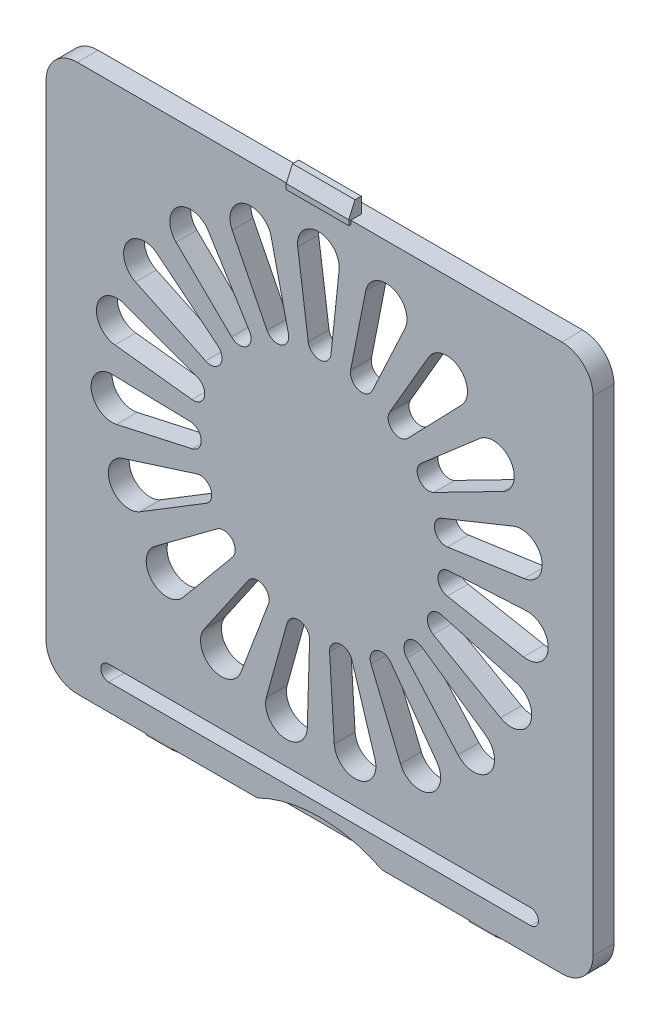
from build123d import *

# Parameters (mm, degrees)
BOSS_EXTRUDE1_DEPTH = 2
CUT_EXTRUDE1_DEPTH  = 12
CUT_EXTRUDE2_START  = -1
SKETCH3_R           = 13.5
CUT_EXTRUDE2_DEPTH  = 1
BOSS_EXTRUDE2_START = 14.25
BOSS_EXTRUDE2_DEPTH = 2.5
BOSS_EXTRUDE3_DEPTH = 3


with BuildPart() as part:
    # Sketch1 → Boss-Extrude1 (new body)
    with BuildSketch(Plane.XY):
        with BuildLine():
            Line((-23.25, 26.25), (23.25, 26.25))
            ThreePointArc((23.25, 26.25), (25.371320344, 25.371320344), (26.25, 23.25))
            Line((26.25, 23.25), (26.25, -23.25))
            ThreePointArc((26.25, -23.25), (25.371320344, -25.371320344), (23.25, -26.25))
            Line((23.25, -26.25), (-23.25, -26.25))
            ThreePointArc((-23.25, -26.25), (-25.371320344, -25.371320344), (-26.25, -23.25))
            Line((-26.25, -23.25), (-26.25, 23.25))
            ThreePointArc((-26.25, 23.25), (-25.371320344, 25.371320344), (-23.25, 26.25))
        make_face()
    extrude(amount=BOSS_EXTRUDE1_DEPTH)

    # Sketch2 → Cut-Extrude1 (cut)
    with BuildSketch(Plane.XY.offset(2)):
        with BuildLine():
            Line((-20.25, -22.25), (20.25, -22.25))
            ThreePointArc((20.25, -22.25), (21, -23), (20.25, -23.75))
            Line((20.25, -23.75), (-20.25, -23.75))
            ThreePointArc((-20.25, -23.75), (-21, -23), (-20.25, -22.25))
        make_face()
        with BuildLine():
            Line((-2.094440492, 21.480216096), (-1.089946345, 14.101618853))
            ThreePointArc((-1.089946345, 14.101618853), (0.01653038, 13.150124213), (1.093913188, 14.134440766))
            Line((1.093913188, 14.134440766), (1.876213205, 21.539892302))
            ThreePointArc((1.876213205, 21.539892302), (-0.1427751, 23.749774158), (-2.094440492, 21.480216096))
        make_face()
        with BuildLine():
            Line((4.425432765, 21.091242282), (2.97967404, 13.786279074))
            ThreePointArc((2.97967404, 13.786279074), (3.717248999, 12.527066633), (5.055863298, 13.108224574))
            Line((5.055863298, 13.108224574), (8.200322325, 19.858415919))
            ThreePointArc((8.200322325, 19.858415919), (7.00827584, 22.604124711), (4.425432765, 21.091242282))
        make_face()
        with BuildLine():
            Line((10.465741714, 18.606344756), (6.726400508, 12.166621695))
            ThreePointArc((6.726400508, 12.166621695), (7.01514601, 10.736146659), (8.469932169, 10.851168508))
            Line((8.469932169, 10.851168508), (13.635799279, 16.21461169))
            ThreePointArc((13.635799279, 16.21461169), (13.399871349, 19.198607267), (10.465741714, 18.606344756))
        make_face()
        with BuildLine():
            Line((15.371925155, 14.294800723), (9.74421711, 9.418161725))
            ThreePointArc((9.74421711, 9.418161725), (9.5528431, 7.971438261), (10.966152465, 7.607859615))
            Line((10.966152465, 7.607859615), (17.593625801, 11.003342342))
            ThreePointArc((17.593625801, 11.003342342), (18.339382876, 13.902262483), (15.371925155, 14.294800723))
        make_face()
        with BuildLine():
            Line((18.612321986, 8.623832879), (11.706096591, 5.838737448))
            ThreePointArc((11.706096591, 5.838737448), (11.055341412, 4.532540491), (12.274019984, 3.729760739))
            Line((12.274019984, 3.729760739), (19.644909973, 4.789329772))
            ThreePointArc((19.644909973, 4.789329772), (21.291537704, 7.289031496), (18.612321986, 8.623832879))
        make_face()
        with BuildLine():
            Line((19.83578493, 2.207978584), (12.399438868, 1.816235025))
            ThreePointArc((12.399438868, 1.816235025), (11.359821941, 0.792111284), (12.251806987, -0.362875933))
            Line((12.251806987, -0.362875933), (19.567363328, -1.754041339))
            ThreePointArc((19.567363328, -1.754041339), (21.93642405, 0.0755605), (19.83578493, 2.207978584))
        make_face()
        with BuildLine():
            Line((18.909732793, -4.257504797), (11.749109546, -2.21344499))
            ThreePointArc((11.749109546, -2.21344499), (10.433289497, -2.844515818), (10.901920596, -4.226549712))
            Line((10.901920596, -4.226549712), (17.369389247, -7.917695201))
            ThreePointArc((17.369389247, -7.917695201), (20.204158471, -6.956458994), (18.909732793, -4.257504797))
        make_face()
        with BuildLine():
            Line((15.934517692, -10.071981817), (9.825581899, -5.813624241))
            ThreePointArc((9.825581899, -5.813624241), (8.376148247, -5.98325584), (8.370641949, -7.442571595))
            Line((8.370641949, -7.442571595), (13.289172328, -13.033704277))
            ThreePointArc((13.289172328, -13.033704277), (16.282458822, -13.044998562), (15.934517692, -10.071981817))
        make_face()
        with BuildLine():
            Line((11.232550351, -14.60536367), (6.837299994, -8.594167444))
            ThreePointArc((6.837299994, -8.594167444), (5.411321364, -8.283977597), (4.932274362, -9.662435707))
            Line((4.932274362, -9.662435707), (7.768867384, -16.547669603))
            ThreePointArc((7.768867384, -16.547669603), (10.596302111, -17.530270468), (11.232550351, -14.60536367))
        make_face()
        with BuildLine():
            Line((5.313361888, -17.36638809), (3.108090542, -10.253759599))
            ThreePointArc((3.108090542, -10.253759599), (1.860093847, -9.497362189), (0.959418316, -10.645585329))
            Line((0.959418316, -10.645585329), (1.406685112, -18.078798509))
            ThreePointArc((1.406685112, -18.078798509), (3.761871648, -19.926225904), (5.313361888, -17.36638809))
        make_face()
        with BuildLine():
            Line((-1.181611781, -18.055855239), (-0.957928747, -10.612558143))
            ThreePointArc((-0.957928747, -10.612558143), (-1.892703701, -9.491920567), (-3.117405592, -10.285480943))
            Line((-3.117405592, -10.285480943), (-5.107933318, -17.461169421))
            ThreePointArc((-5.107933318, -17.461169421), (-3.48021598, -19.973225922), (-1.181611781, -18.055855239))
        make_face()
        with BuildLine():
            Line((-7.548539479, -16.599050654), (-4.920141592, -9.631681687))
            ThreePointArc((-4.920141592, -9.631681687), (-5.440397435, -8.268242415), (-6.856410232, -8.621145447))
            Line((-6.856410232, -8.621145447), (-11.069027916, -14.761712035))
            ThreePointArc((-11.069027916, -14.761712035), (-10.345168205, -17.666177341), (-7.548539479, -16.599050654))
        make_face()
        with BuildLine():
            Line((-13.097465797, -13.153841715), (-8.349180752, -7.417423416))
            ThreePointArc((-8.349180752, -7.417423416), (-8.39853969, -5.958932248), (-9.852416435, -5.832935417))
            Line((-9.852416435, -5.832935417), (-15.830621585, -10.272954444))
            ThreePointArc((-15.830621585, -10.272954444), (-16.089060933, -13.255084672), (-13.097465797, -13.153841715))
        make_face()
        with BuildLine():
            Line((-17.227078467, -8.09357027), (-10.873456626, -4.209732571))
            ThreePointArc((-10.873456626, -4.209732571), (-10.446569853, -2.814239656), (-11.780760442, -2.222996673))
            Line((-11.780760442, -2.222996673), (-18.876721768, -4.481323183))
            ThreePointArc((-18.876721768, -4.481323183), (-20.089454262, -7.217958251), (-17.227078467, -8.09357027))
        make_face()
        with BuildLine():
            Line((-19.48986988, -1.966595247), (-12.219424756, -0.356212226))
            ThreePointArc((-12.219424756, -0.356212226), (-11.362552077, 0.825059124), (-12.432476257, 1.817477908))
            Line((-12.432476257, 1.817477908), (-19.877236245, 1.985568633))
            ThreePointArc((-19.877236245, 1.985568633), (-21.912843501, -0.209014401), (-19.48986988, -1.966595247))
        make_face()
        with BuildLine():
            Line((-19.640631475, 4.56313054), (-12.24122861, 3.725548894))
            ThreePointArc((-12.24122861, 3.725548894), (-11.047225476, 4.564589601), (-11.73694036, 5.85064021))
            Line((-11.73694036, 5.85064021), (-18.723743748, 8.426932933))
            ThreePointArc((-18.723743748, 8.426932933), (-21.361636134, 7.012219056), (-19.640631475, 4.56313054))
        make_face()
        with BuildLine():
            Line((-17.663025894, 10.788009983), (-10.936505402, 7.593228638))
            ThreePointArc((-10.936505402, 7.593228638), (-9.534760578, 7.999115621), (-9.769524858, 9.439434518))
            Line((-9.769524858, 9.439434518), (-15.541243087, 14.144747946))
            ThreePointArc((-15.541243087, 14.144747946), (-18.495564033, 13.663209427), (-17.663025894, 10.788009983))
        make_face()
        with BuildLine():
            Line((-13.771357387, 16.033480805), (-8.446642136, 10.827703892))
            ThreePointArc((-8.446642136, 10.827703892), (-6.989056426, 10.756452998), (-6.743429747, 12.194959282))
            Line((-6.743429747, 12.194959282), (-10.67460759, 18.519399695))
            ThreePointArc((-10.67460759, 18.519399695), (-13.625210579, 19.023218704), (-13.771357387, 16.033480805))
        make_face()
        with BuildLine():
            Line((-8.387348622, 19.73111485), (-5.041454131, 13.078469074))
            ThreePointArc((-5.041454131, 13.078469074), (-3.685979563, 12.537801444), (-2.986579389, 13.818610637))
            Line((-2.986579389, 13.818610637), (-4.651212727, 21.076826783))
            ThreePointArc((-4.651212727, 21.076826783), (-7.278354143, 22.511406713), (-8.387348622, 19.73111485))
        make_face()
    extrude(amount=-CUT_EXTRUDE1_DEPTH, mode=Mode.SUBTRACT)

    # Sketch3 → Cut-Extrude2 (cut)
    with BuildSketch(Plane(origin=(0, 0, 0), x_dir=(-1, 0, 0), z_dir=(0, 0, -1)).offset(CUT_EXTRUDE2_START)):
        with Locations((0, -38.352973417)):
            Circle(SKETCH3_R)
    extrude(amount=-CUT_EXTRUDE2_DEPTH, mode=Mode.SUBTRACT)

    # Sketch4 → Boss-Extrude2 (add)
    with BuildSketch(Plane(origin=(0, 0, 0), x_dir=(0, 0, -1), z_dir=(1, 0, 0)).offset(BOSS_EXTRUDE2_START)):
        Polygon((-1, -26.25), (-1, -27), (-1.25, -27), (-1.892304423, -26.45), (-1.892304423, -26.25), align=None)
    boss_extrude2 = extrude(amount=BOSS_EXTRUDE2_DEPTH)

    # Mirror3: Boss-Extrude2 across plane
    add(boss_extrude2.mirror(Plane(origin=(0, 0, 0), x_dir=(0, 0, 1), z_dir=(1, 0, 0))))

    # Sketch5 → Boss-Extrude3 (add, symmetric)
    with BuildSketch(Plane(origin=(0, 0, 0), x_dir=(0, 0, -1), z_dir=(1, 0, 0))):
        Polygon((-1, 26.25), (-1, 27.75), (-1.6, 27.75), (-2.2, 26.392012559), (-2.2, 25.892012559), (-1, 25.892012559), align=None)
    extrude(amount=BOSS_EXTRUDE3_DEPTH, both=True)


solid = part.part
